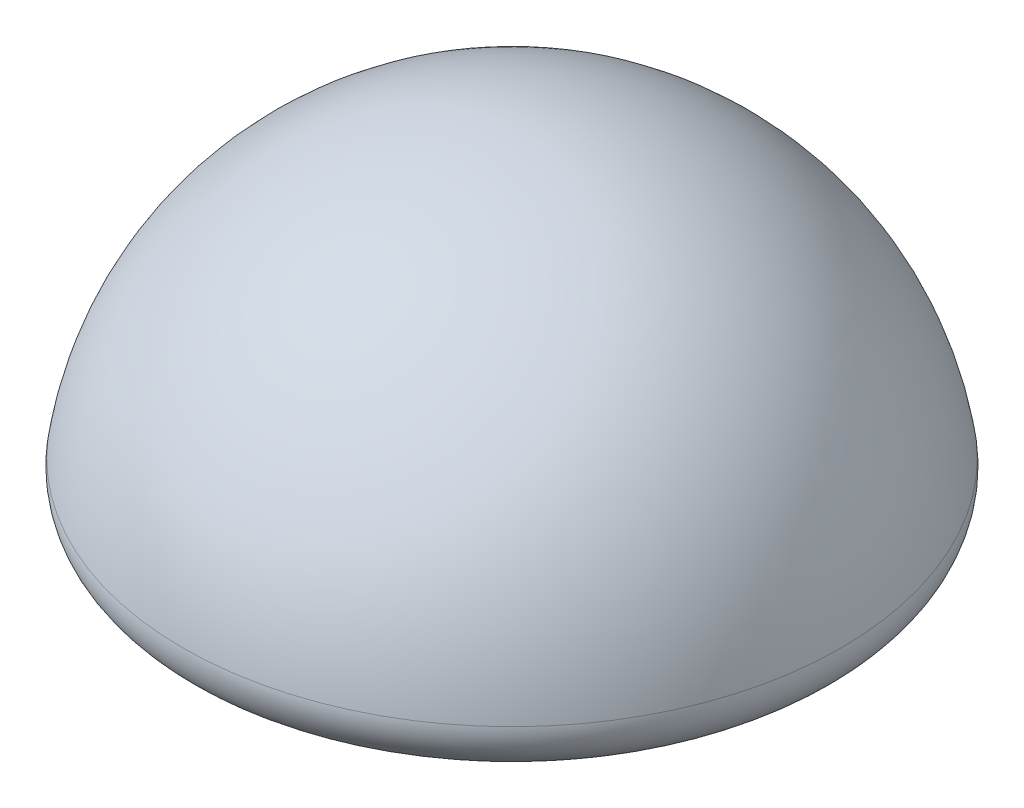
SolidWorks part; units mm, degrees
ref_plane "前视基准面" through (0, 0, 0) normal (0, 0, 1) x (1, 0, 0)
ref_plane "上视基准面" through (0, 0, 0) normal (0, 1, 0) x (1, 0, 0)
ref_plane "右视基准面" through (0, 0, 0) normal (1, 0, 0) x (0, 0, -1)
sketch "草图1" plane through (0, 0, 0) normal (0, 0, 1) x (1, 0, 0)
  line L0 (0, 0) -> (15, 0)
  line L1 (0, 0) -> (0, 19.2874)
  circle A0 centre (0, 0) radius 15
  dimension "D1" = 30
revolve "旋转1" add sketch "草图1" angle 360 about L1
sketch "草图2" plane through (0, 0, 0) normal (0, -1, 0) x (1, 0, 0)
  circle A0 centre (0, 0) radius 5
  dimension "D1" = 10
extrude "凸台-拉伸1" add sketch "草图2" along normal blind 2
fillet "圆角1" radius 2 1 edges at (0, 0, -15)
